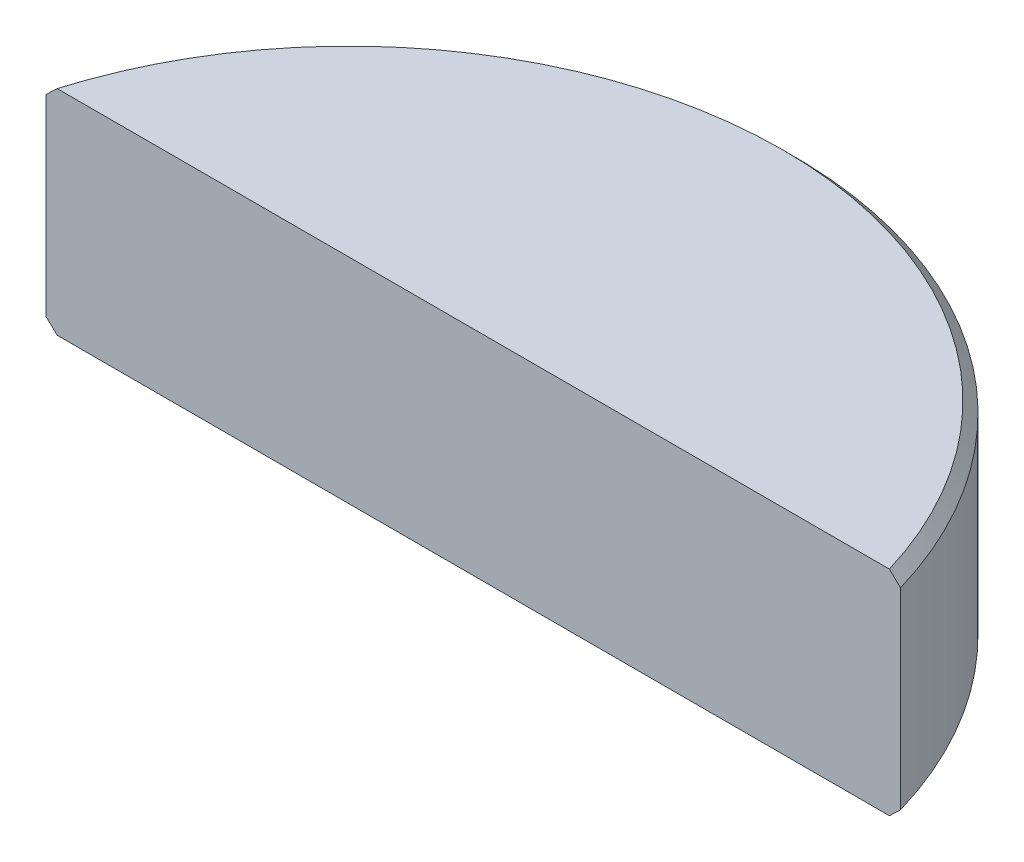
from build123d import *

# Parameters (mm, degrees)
BOSS_EXTRUDE1_DEPTH = 6
CHAMFER1_SIZE       = 0.3


with BuildPart() as part:
    # Sketch1 → Boss-Extrude1 (new body)
    with BuildSketch(Plane.XZ.offset(3)):
        with BuildLine():
            Line((12, 0), (-12, 0))
            ThreePointArc((-12, 0), (0, -9), (12, 0))
        make_face()
    extrude(amount=-BOSS_EXTRUDE1_DEPTH)

    # Chamfer1
    chamfer1_edges = [part.edges().sort_by_distance(p)[0] for p in [
        (0, -3, -9),
        (0, 3, -9),
    ]]
    chamfer(chamfer1_edges, length=CHAMFER1_SIZE)


solid = part.part
